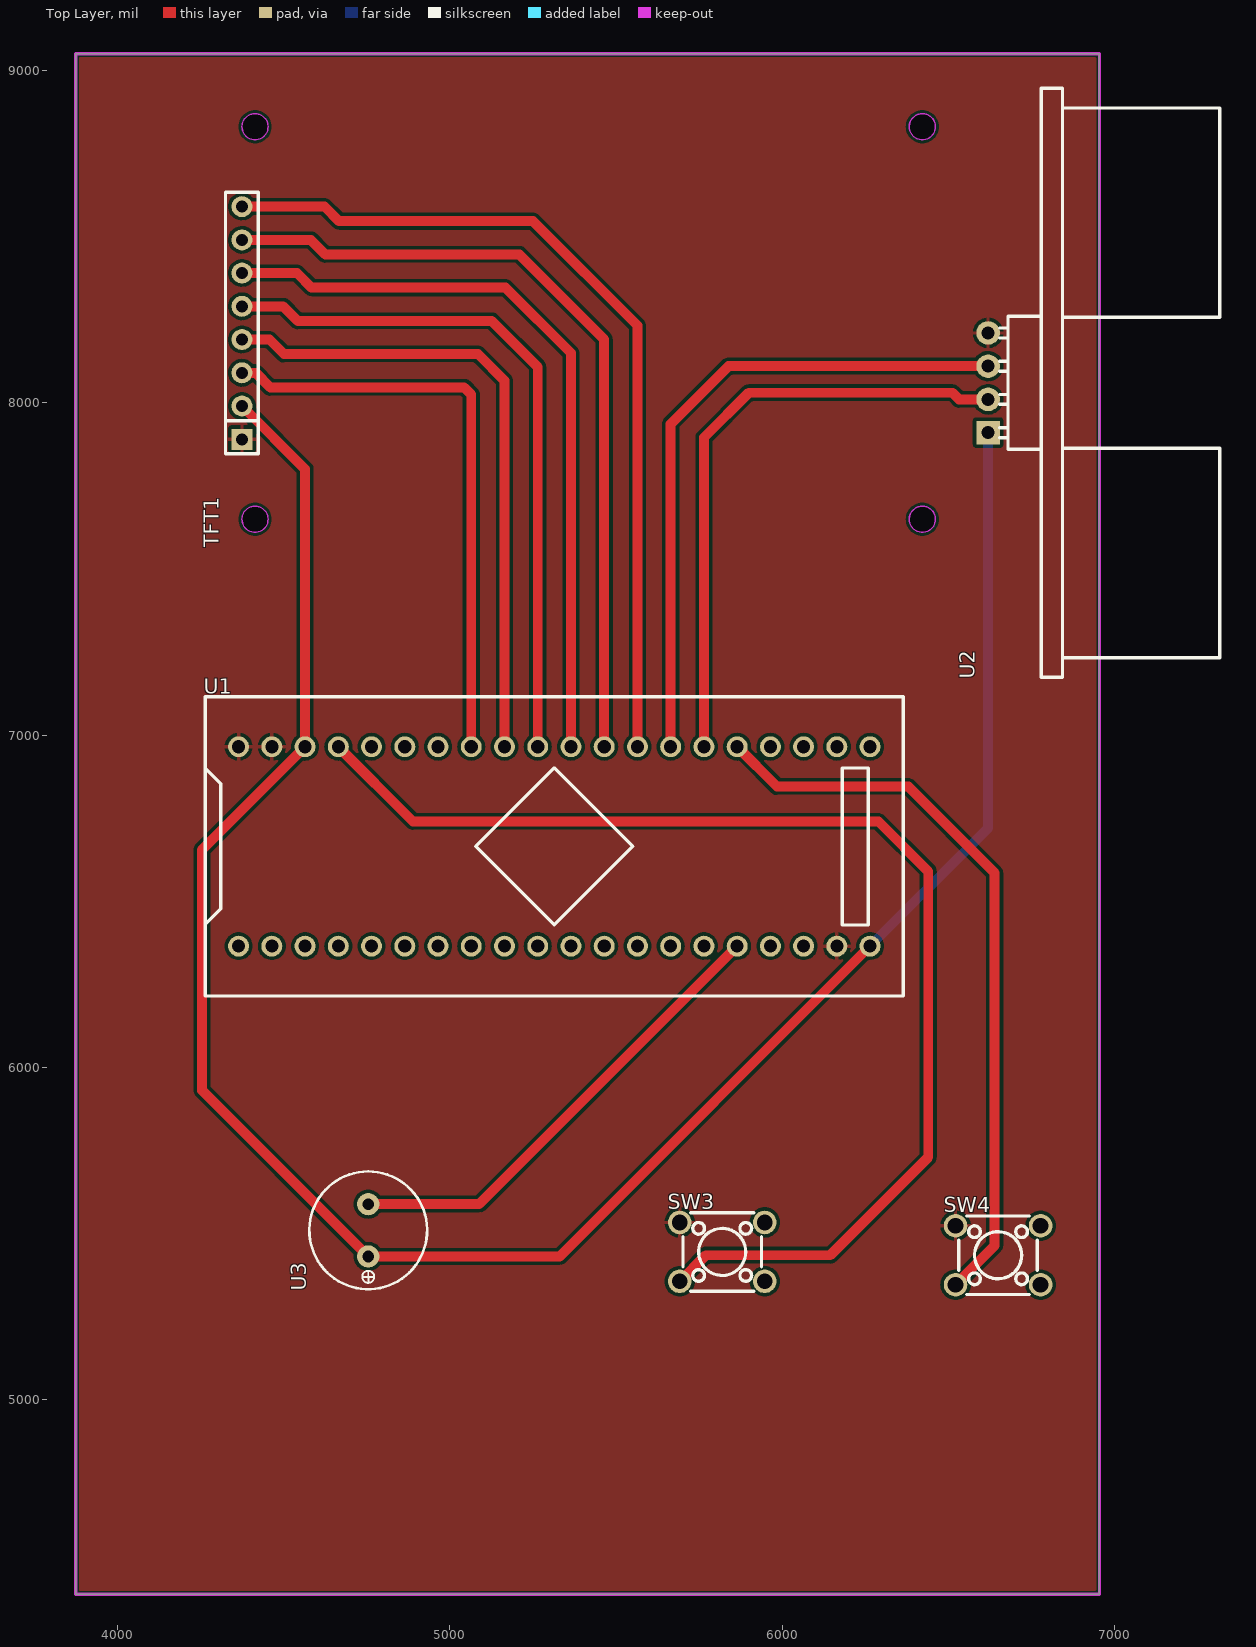
[diagram p0: Top Layer view]
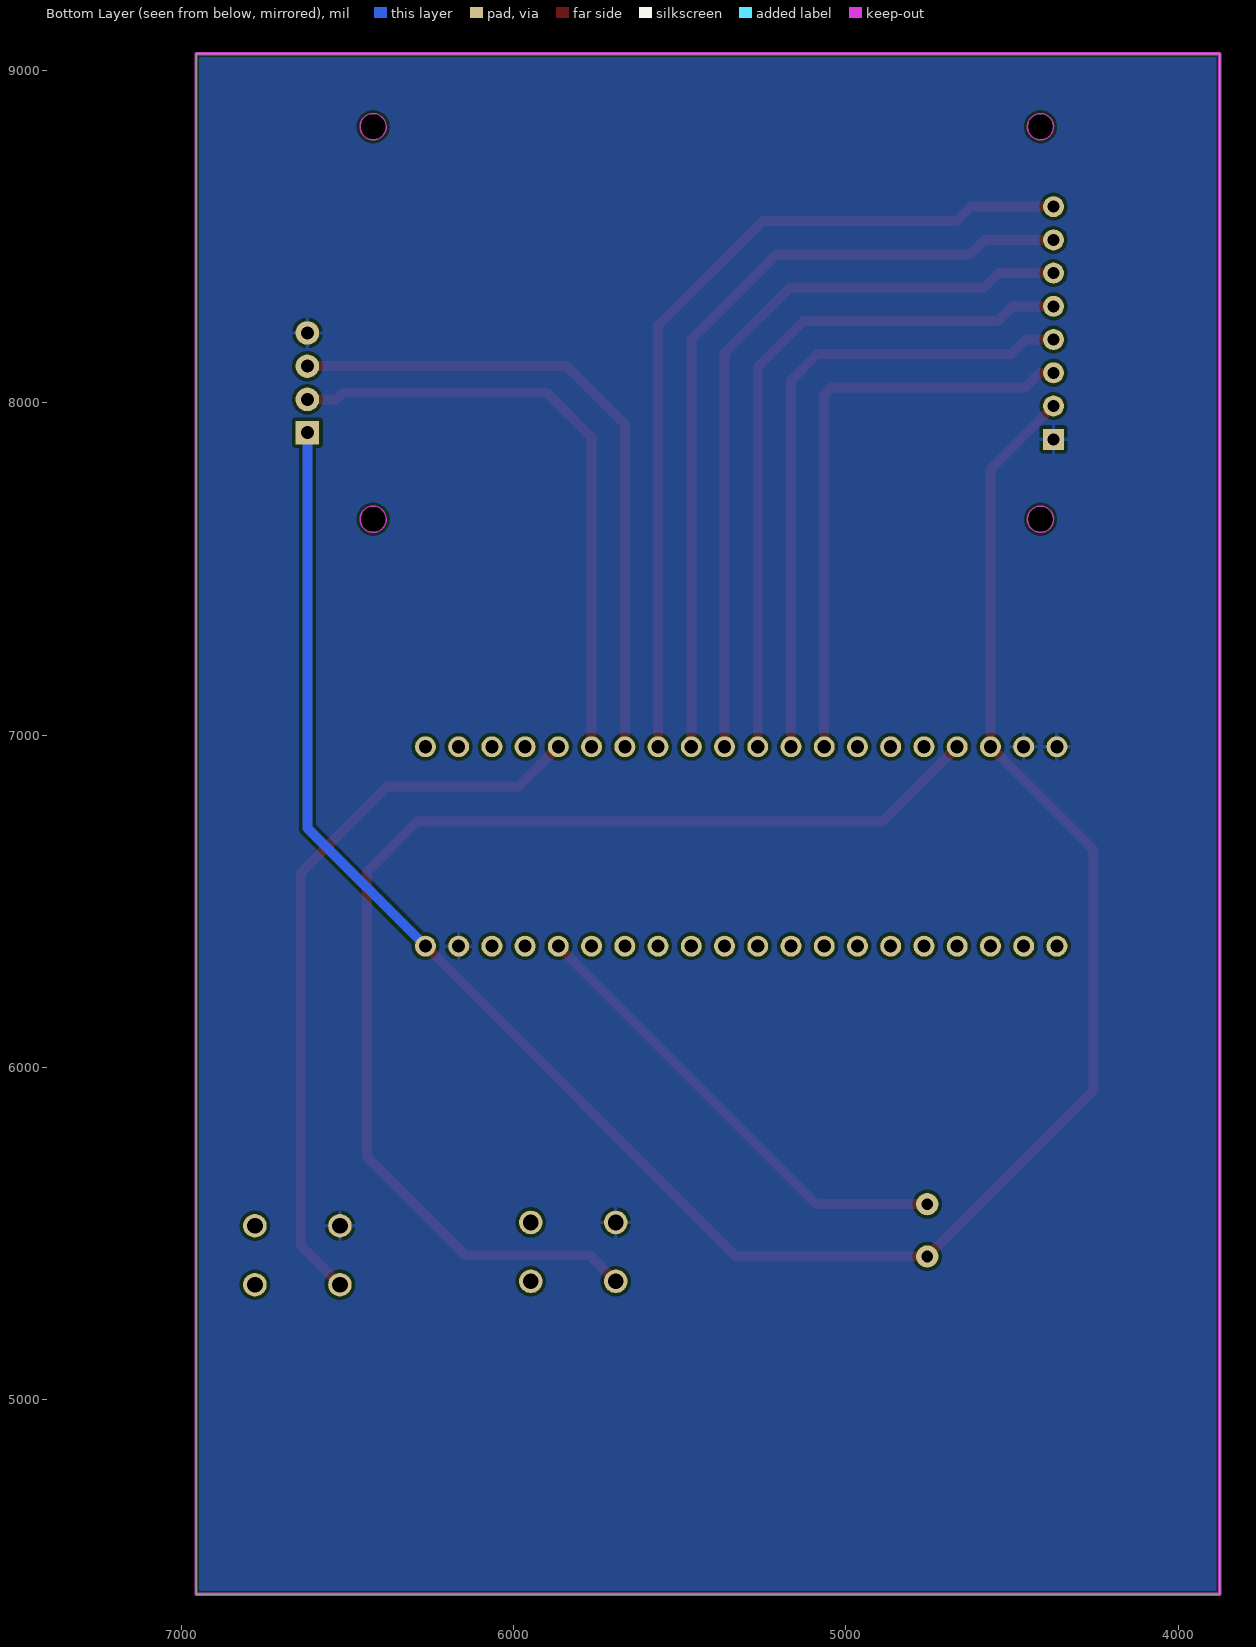
[diagram p1: Bottom Layer view, seen from below]
# Altium PCB MISC49920.pcbdoc
Units mil, origin at the board's own origin, x right, y up, seen from the top; angles counter-clockwise.
Board outline 3080 x 4635 mil, 2 copper layers (Top Layer, Bottom Layer), stack 62.206 mil thick; 6 components, 37 nets, 62 pads, 0 vias.

## Layer stack, top to bottom
Top Solder Mask Layer: solder mask 0.394, Dk 3.3
Top Layer: signal copper 1.379
Dielectric1: surface 59.449, FR4, Dk 4.5
Bottom Layer: signal copper 1.378
Bottom Solder Mask Layer: solder mask 0.394, Dk 3.3

## Board outline
3875,9050 3875,4415 6955,4415 6955,9050

## Design rules (kind name [scope] priority, off if disabled: settings)
BoardOutlineClearance copperThickness2oz_1 [All] p2 off: genericclearance=7.99 ignorepadtopadclearanceinfootprint=FALSE except(0: Arc-SplitContinuation Track-SplitContinuation SMDPad-SplitContinuation THPad-SplitContinuation Via-SplitContinuation Fill-SplitContinuation Region-SplitContinuation Poly-SplitContinuation Text-SplitContinuation Hole-SplitContinuation; 5.98: Arc-CutoutEdge Track-CutoutEdge SMDPad-CutoutEdge THPad-CutoutEdge Via-CutoutEdge Text-CutoutEdge; 6.9: Hole-OutlineEdge Hole-CutoutEdge; 10: Poly-OutlineEdge Poly-CutoutEdge; 11.81: Arc-OutlineEdge Track-OutlineEdge SMDPad-OutlineEdge THPad-OutlineEdge Via-OutlineEdge Fill-OutlineEdge Region-OutlineEdge Text-OutlineEdge Fill-CutoutEdge Region-CutoutEdge)
BoardOutlineClearance Plane_innerPlane_1 [All] p4 off: genericclearance=4.02 ignorepadtopadclearanceinfootprint=FALSE except(0: Arc-SplitContinuation Track-SplitContinuation SMDPad-SplitContinuation THPad-SplitContinuation Via-SplitContinuation Fill-SplitContinuation Region-SplitContinuation Poly-SplitContinuation Text-SplitContinuation Hole-SplitContinuation; 5.98: Arc-CutoutEdge Track-CutoutEdge SMDPad-CutoutEdge THPad-CutoutEdge Via-CutoutEdge Text-CutoutEdge; 6.9: Hole-OutlineEdge Hole-CutoutEdge; 10: Poly-OutlineEdge Poly-CutoutEdge; 11.81: Arc-OutlineEdge Track-OutlineEdge SMDPad-OutlineEdge THPad-OutlineEdge Via-OutlineEdge Fill-OutlineEdge Region-OutlineEdge Text-OutlineEdge Fill-CutoutEdge Region-CutoutEdge)
BoardOutlineClearance Copper_copperRegion_1 [All] p6 off: genericclearance=4.02 ignorepadtopadclearanceinfootprint=FALSE except(0: Arc-SplitContinuation Track-SplitContinuation SMDPad-SplitContinuation THPad-SplitContinuation Via-SplitContinuation Fill-SplitContinuation Region-SplitContinuation Poly-SplitContinuation Text-SplitContinuation Hole-SplitContinuation; 5.98: Arc-CutoutEdge Track-CutoutEdge SMDPad-CutoutEdge THPad-CutoutEdge Via-CutoutEdge Text-CutoutEdge; 6.9: Hole-OutlineEdge Hole-CutoutEdge; 10: Poly-OutlineEdge Poly-CutoutEdge; 11.81: Arc-OutlineEdge Track-OutlineEdge SMDPad-OutlineEdge THPad-OutlineEdge Via-OutlineEdge Fill-OutlineEdge Region-OutlineEdge Text-OutlineEdge Fill-CutoutEdge Region-CutoutEdge)
BoardOutlineClearance Copper_copperRegion_copperThickness1oz_1 [All] p8 off: genericclearance=4.02 ignorepadtopadclearanceinfootprint=FALSE except(0: Arc-SplitContinuation Track-SplitContinuation SMDPad-SplitContinuation THPad-SplitContinuation Via-SplitContinuation Fill-SplitContinuation Region-SplitContinuation Poly-SplitContinuation Text-SplitContinuation Hole-SplitContinuation; 5.98: Arc-CutoutEdge Track-CutoutEdge SMDPad-CutoutEdge THPad-CutoutEdge Via-CutoutEdge Text-CutoutEdge; 6.9: Hole-OutlineEdge Hole-CutoutEdge; 10: Poly-OutlineEdge Poly-CutoutEdge; 11.81: Arc-OutlineEdge Track-OutlineEdge SMDPad-OutlineEdge THPad-OutlineEdge Via-OutlineEdge Fill-OutlineEdge Region-OutlineEdge Text-OutlineEdge Fill-CutoutEdge Region-CutoutEdge)
BoardOutlineClearance Copper_copperRegion_Copper_copperRegion_1 [All] p10 off: genericclearance=4.02 ignorepadtopadclearanceinfootprint=FALSE except(0: Arc-SplitContinuation Track-SplitContinuation SMDPad-SplitContinuation THPad-SplitContinuation Via-SplitContinuation Fill-SplitContinuation Region-SplitContinuation Poly-SplitContinuation Text-SplitContinuation Hole-SplitContinuation; 5.98: Arc-CutoutEdge Track-CutoutEdge SMDPad-CutoutEdge THPad-CutoutEdge Via-CutoutEdge Text-CutoutEdge; 6.9: Hole-OutlineEdge Hole-CutoutEdge; 10: Poly-OutlineEdge Poly-CutoutEdge; 11.81: Arc-OutlineEdge Track-OutlineEdge SMDPad-OutlineEdge THPad-OutlineEdge Via-OutlineEdge Fill-OutlineEdge Region-OutlineEdge Text-OutlineEdge Fill-CutoutEdge Region-CutoutEdge)
BoardOutlineClearance copperThickness1oz_1 [All] p12: genericclearance=4.02 ignorepadtopadclearanceinfootprint=FALSE except(0: Arc-SplitContinuation Track-SplitContinuation SMDPad-SplitContinuation THPad-SplitContinuation Via-SplitContinuation Fill-SplitContinuation Region-SplitContinuation Poly-SplitContinuation Text-SplitContinuation Hole-SplitContinuation; 5.98: Arc-CutoutEdge Track-CutoutEdge SMDPad-CutoutEdge THPad-CutoutEdge Via-CutoutEdge Text-CutoutEdge; 6.9: Hole-OutlineEdge Hole-CutoutEdge; 10: Poly-OutlineEdge Poly-CutoutEdge; 11.81: Arc-OutlineEdge Track-OutlineEdge SMDPad-OutlineEdge THPad-OutlineEdge Via-OutlineEdge Fill-OutlineEdge Region-OutlineEdge Text-OutlineEdge Fill-CutoutEdge Region-CutoutEdge)
Clearance copperThickness2oz [All] p1 off: gap=7.99 ignorepadtopadclearanceinfootprint=FALSE except(5.98: SMDPad-Track SMDPad-SMDPad THPad-Track SMDPad-THPad THPad-THPad Track-Via SMDPad-Via THPad-Via Via-Via Fill-SMDPad Region-SMDPad Fill-THPad Region-THPad Fill-Via Region-Via Fill-Fill Fill-Region Region-Region Arc-Track Arc-SMDPad Arc-THPad Arc-Via Fill-Arc Region-Arc Arc-Arc Text-Track SMDPad-Text Text-THPad Text-Via Fill-Text Region-Text Arc-Text Text-Text; 6.9: Hole-Track Hole-SMDPad Hole-THPad Hole-Via Fill-Hole Region-Hole Hole-Arc Hole-Text; 10: Poly-Track Poly-SMDPad Poly-THPad Poly-Via Poly-Fill Poly-Region Poly-Poly Poly-Arc Poly-Text Poly-Hole; 11.81: Fill-Track Region-Track)
Clearance Plane_innerPlane [All] p3 off: gap=4.02 ignorepadtopadclearanceinfootprint=FALSE except(5.98: SMDPad-Track SMDPad-SMDPad THPad-Track SMDPad-THPad THPad-THPad Track-Via SMDPad-Via THPad-Via Via-Via Fill-SMDPad Region-SMDPad Fill-THPad Region-THPad Fill-Via Region-Via Fill-Fill Fill-Region Region-Region Arc-Track Arc-SMDPad Arc-THPad Arc-Via Fill-Arc Region-Arc Arc-Arc Text-Track SMDPad-Text Text-THPad Text-Via Fill-Text Region-Text Arc-Text Text-Text; 6.9: Hole-Track Hole-SMDPad Hole-THPad Hole-Via Fill-Hole Region-Hole Hole-Arc Hole-Text; 10: Poly-Track Poly-SMDPad Poly-THPad Poly-Via Poly-Fill Poly-Region Poly-Poly Poly-Arc Poly-Text Poly-Hole; 11.81: Fill-Track Region-Track)
Clearance Copper_copperRegion [All] p5 off: gap=4.02 ignorepadtopadclearanceinfootprint=FALSE except(5.98: SMDPad-Track SMDPad-SMDPad THPad-Track SMDPad-THPad THPad-THPad Track-Via SMDPad-Via THPad-Via Via-Via Fill-SMDPad Region-SMDPad Fill-THPad Region-THPad Fill-Via Region-Via Fill-Fill Fill-Region Region-Region Arc-Track Arc-SMDPad Arc-THPad Arc-Via Fill-Arc Region-Arc Arc-Arc Text-Track SMDPad-Text Text-THPad Text-Via Fill-Text Region-Text Arc-Text Text-Text; 6.9: Hole-Track Hole-SMDPad Hole-THPad Hole-Via Fill-Hole Region-Hole Hole-Arc Hole-Text; 10: Poly-Track Poly-SMDPad Poly-THPad Poly-Via Poly-Fill Poly-Region Poly-Poly Poly-Arc Poly-Text Poly-Hole; 11.81: Fill-Track Region-Track)
Clearance Copper_copperRegion_copperThickness1oz [All] p7 off: gap=4.02 ignorepadtopadclearanceinfootprint=FALSE except(5.98: SMDPad-Track SMDPad-SMDPad THPad-Track SMDPad-THPad THPad-THPad Track-Via SMDPad-Via THPad-Via Via-Via Fill-SMDPad Region-SMDPad Fill-THPad Region-THPad Fill-Via Region-Via Fill-Fill Fill-Region Region-Region Arc-Track Arc-SMDPad Arc-THPad Arc-Via Fill-Arc Region-Arc Arc-Arc Text-Track SMDPad-Text Text-THPad Text-Via Fill-Text Region-Text Arc-Text Text-Text; 6.9: Hole-Track Hole-SMDPad Hole-THPad Hole-Via Fill-Hole Region-Hole Hole-Arc Hole-Text; 10: Poly-Track Poly-SMDPad Poly-THPad Poly-Via Poly-Fill Poly-Region Poly-Poly Poly-Arc Poly-Text Poly-Hole; 11.81: Fill-Track Region-Track)
Clearance Copper_copperRegion_Copper_copperRegion [All] p9 off: gap=4.02 ignorepadtopadclearanceinfootprint=FALSE except(5.98: SMDPad-Track SMDPad-SMDPad THPad-Track SMDPad-THPad THPad-THPad Track-Via SMDPad-Via THPad-Via Via-Via Fill-SMDPad Region-SMDPad Fill-THPad Region-THPad Fill-Via Region-Via Fill-Fill Fill-Region Region-Region Arc-Track Arc-SMDPad Arc-THPad Arc-Via Fill-Arc Region-Arc Arc-Arc Text-Track SMDPad-Text Text-THPad Text-Via Fill-Text Region-Text Arc-Text Text-Text; 6.9: Hole-Track Hole-SMDPad Hole-THPad Hole-Via Fill-Hole Region-Hole Hole-Arc Hole-Text; 10: Poly-Track Poly-SMDPad Poly-THPad Poly-Via Poly-Fill Poly-Region Poly-Poly Poly-Arc Poly-Text Poly-Hole; 11.81: Fill-Track Region-Track)
Clearance copperThickness1oz [All] p11: gap=4.02 ignorepadtopadclearanceinfootprint=FALSE except(5.98: SMDPad-Track SMDPad-SMDPad THPad-Track SMDPad-THPad THPad-THPad Track-Via SMDPad-Via THPad-Via Via-Via Fill-SMDPad Region-SMDPad Fill-THPad Region-THPad Fill-Via Region-Via Fill-Fill Fill-Region Region-Region Arc-Track Arc-SMDPad Arc-THPad Arc-Via Fill-Arc Region-Arc Arc-Arc Text-Track SMDPad-Text Text-THPad Text-Via Fill-Text Region-Text Arc-Text Text-Text; 6.9: Hole-Track Hole-SMDPad Hole-THPad Hole-Via Fill-Hole Region-Hole Hole-Arc Hole-Text; 10: Poly-Track Poly-SMDPad Poly-THPad Poly-Via Poly-Fill Poly-Region Poly-Poly Poly-Arc Poly-Text Poly-Hole; 11.81: Fill-Track Region-Track)
DiffPairsRouting differentialPair [All] p1: maxlimit=6 minlimit=6 mostfreqgap=6 toplayer_minwidth=5 toplayer_prefwidth=10 toplayer_maxwidth=100 toplayer_mingap=6 toplayer_prefgap=6 toplayer_maxgap=6 bottomlayer_minwidth=5 bottomlayer_prefwidth=10 bottomlayer_maxwidth=100 bottomlayer_mingap=6 bottomlayer_prefgap=6 bottomlayer_maxgap=6 maxuncoupledlength=10
HoleToHoleClearance otherClearance [All] p1: gap=11.81 allowstackedmicrovias=TRUE
Length netLength [All] p1: minlimit=0 maxlimit=0
PasteMaskExpansion pasteMaskExpansion [All] p1: expansion=0
PlaneConnect innerPlane [All] p1: planeconnectstyle=Relief reliefexpansion=20 reliefentries=4 reliefconductorwidth=10 reliefairgap=10
PolygonConnect copperRegion_copperThickness1oz [(InNet('GND'))] p1: connectstyle=Relief reliefconductorwidth=10 reliefentries=4 polygonreliefangle="90 Angle" airgapwidth=10 via.connectstyle=Relief via.reliefconductorwidth=10 via.reliefentries=4 via.polygonreliefangle="90 Angle" via.airgapwidth=10
PolygonConnect copperRegion_Copper_copperRegion [All] p2 off: connectstyle=Relief reliefconductorwidth=10 reliefentries=4 polygonreliefangle="90 Angle" airgapwidth=10 via.connectstyle=Relief via.reliefconductorwidth=10 via.reliefentries=4 via.polygonreliefangle="90 Angle" via.airgapwidth=10
PolygonConnect copperRegion [All] p3: connectstyle=Relief reliefconductorwidth=10 reliefentries=4 polygonreliefangle="90 Angle" airgapwidth=10 via.connectstyle=Relief via.reliefconductorwidth=10 via.reliefentries=4 via.polygonreliefangle="90 Angle" via.airgapwidth=10
RoutingVias viaSize [All] p1: holewidth=12.01 width=24.02 viastyle="Through Hole" minholewidth=11.81 minwidth=19.68 maxholewidth=248.03 maxwidth=393.7
SolderMaskExpansion solderMaskExpansion [IsVia] p1: expansion=-1000 istentingtop=TRUE
SolderMaskExpansion solderMaskExpansion [All] p2: expansion=2 istentingtop=FALSE
Width copperThickness2oz_2 [All] p1 off: maxlimit=100 minlimit=8 preferedwidth=10
Width copperThickness1oz_2 [All] p2: maxlimit=100 minlimit=5 preferedwidth=10

## Components (designator, comment, footprint, x,y, rotation, side; value= is the part's Value field where it differs from the comment)
SW3 "" SW-TH_4P-L6.0-W6.0-P4.50-LS6.5 5820,5445 r0 top
SW4 "" SW-TH_4P-L6.0-W6.0-P4.50-LS6.5 6650,5435 r0 top
TFT1 "1.8 TFT 128*RGB*160" LCD-TH_8P-P2.54-L56.0-W34.0_1.8-TFT 4375,8240 r90 top
U1 "STM32F103C8T6-Card" CONN-TH_L53.3-W22.9_STM32F103C8T6-CARD 5315,6665 r0 top
U2 "HC-SR04" TH_HC-SR04V 6620,8060 r90 top
U3 "CUI_CST-931AP" BUZ-TH_BD9.0-P4.00-D0.6-L-FD 4755,5510 r90 top

## Footprints (in the part's own frame and the unit in brackets; to place one, negate y for a bottom-side part, rotate by r counter-clockwise, add the part's x,y. Pads: shape width x height; smd on the part's side, far side on the other; paste and mask are expansions set on the pad)
BUZ-TH_BD9.0-P4.00-D0.6-L-FD [mm]
  round 1.7 hole 0.9 paste+0 mask+0.05: 1(-2,0) 2(2,0)
  silkscreen extent -4.5,-4.5 4.5,4.5
CONN-TH_L53.3-W22.9_STM32F103C8T6-CARD [mm]
  round 1.6 hole 1: 1(-24.13,-7.62) 2(-21.59,-7.62) 3(-19.05,-7.62) 4(-16.51,-7.62) 5(-13.97,-7.62) 6(-11.43,-7.62) 7(-8.89,-7.62) 8(-6.35,-7.62) 9(-3.81,-7.62) 10(-1.27,-7.62) 11(1.27,-7.62) 12(3.81,-7.62) 13(6.35,-7.62) 14(8.89,-7.62) 15(11.43,-7.62) 16(13.97,-7.62) 17(16.51,-7.62) 18(19.05,-7.62) 19(21.59,-7.62) 20(24.13,-7.62) 21(24.13,7.62) 22(21.59,7.62) 23(19.05,7.62) 24(16.51,7.62) 25(13.97,7.62) 26(11.43,7.62) 27(8.89,7.62) 28(6.35,7.62) 29(3.81,7.62) 30(1.27,7.62) 31(-1.27,7.62) 32(-3.81,7.62) 33(-6.35,7.62) 34(-8.89,7.62) 35(-11.43,7.62) 36(-13.97,7.62) 37(-16.51,7.62) 38(-19.05,7.62) 39(-21.59,7.62) 40(-24.13,7.62)
  silkscreen extent -26.67,-11.43 26.67,11.43
LCD-TH_8P-P2.54-L56.0-W34.0_1.8-TFT [mm]
  rect 1.6x1.6 hole 0.914: 1(-8.89,0)
  round 1.6 hole 0.914: 2(-6.35,0) 3(-3.81,0) 4(-1.27,0) 5(1.27,0) 6(3.81,0) 7(6.35,0) 8(8.89,0)
  Board Outline Layer circle w0.003: c15,-1 r1
  Board Outline Layer circle w0.003: c-15,-1 r1
  Board Outline Layer circle w0.003: c15,-52 r1
  Board Outline Layer circle w0.003: c-15,-52 r1
  Board Outline Layer region: 15,-2 14.566,-1.901 14.218,-1.623 14.025,-1.223 14.025,-0.777 14.218,-0.377 14.566,-0.099 15,0 15,0 15.434,-0.099 15.782,-0.377 15.975,-0.777 15.975,-1.223 15.782,-1.623 15.434,-1.901 15,-2
  Board Outline Layer region: 15,-2 14.864,-1.991 14.73,-1.963 14.602,-1.917 14.48,-1.854 14.369,-1.776 14.269,-1.683 14.183,-1.577 14.112,-1.46 14.058,-1.335 14.021,-1.203 14.002,-1.068 14.002,-0.932 14.021,-0.797 14.058,-0.665 14.112,-0.54 14.183,-0.423 14.269,-0.317 14.369,-0.224 14.48,-0.146 14.602,-0.083 14.73,-0.037 14.864,-0.009 15,0 15.136,-0.009 15.27,-0.037 15.398,-0.083 15.52,-0.146 15.631,-0.224 15.731,-0.317 15.817,-0.423 15.888,-0.54 15.942,-0.665 15.979,-0.797 15.998,-0.932 15.998,-1.068 15.979,-1.203 15.942,-1.335 15.888,-1.46 15.817,-1.577 15.731,-1.683 15.631,-1.776 15.52,-1.854 15.398,-1.917 15.27,-1.963 15.136,-1.991
  Board Outline Layer region: -15,-2 -15.434,-1.901 -15.782,-1.623 -15.975,-1.223 -15.975,-0.777 -15.782,-0.377 -15.434,-0.099 -15,0 -15,0 -14.566,-0.099 -14.218,-0.377 -14.025,-0.777 -14.025,-1.223 -14.218,-1.623 -14.566,-1.901 -15,-2
  Board Outline Layer region: -15,-2 -15.136,-1.991 -15.27,-1.963 -15.398,-1.917 -15.52,-1.854 -15.631,-1.776 -15.731,-1.683 -15.817,-1.577 -15.888,-1.46 -15.942,-1.335 -15.979,-1.203 -15.998,-1.068 -15.998,-0.932 -15.979,-0.797 -15.942,-0.665 -15.888,-0.54 -15.817,-0.423 -15.731,-0.317 -15.631,-0.224 -15.52,-0.146 -15.398,-0.083 -15.27,-0.037 -15.136,-0.009 -15,0 -14.864,-0.009 -14.73,-0.037 -14.602,-0.083 -14.48,-0.146 -14.369,-0.224 -14.269,-0.317 -14.183,-0.423 -14.112,-0.54 -14.058,-0.665 -14.021,-0.797 -14.002,-0.932 -14.002,-1.068 -14.021,-1.203 -14.058,-1.335 -14.112,-1.46 -14.183,-1.577 -14.269,-1.683 -14.369,-1.776 -14.48,-1.854 -14.602,-1.917 -14.73,-1.963 -14.864,-1.991
  Board Outline Layer region: 15,-53 14.566,-52.901 14.218,-52.623 14.025,-52.222 14.025,-51.777 14.218,-51.376 14.566,-51.099 15,-51 15,-51 15.434,-51.099 15.782,-51.376 15.975,-51.777 15.975,-52.222 15.782,-52.623 15.434,-52.901 15,-53
  Board Outline Layer region: 15,-53 14.864,-52.991 14.73,-52.963 14.602,-52.917 14.48,-52.854 14.369,-52.776 14.269,-52.682 14.183,-52.577 14.112,-52.46 14.058,-52.335 14.021,-52.203 14.002,-52.068 14.002,-51.932 14.021,-51.796 14.058,-51.665 14.112,-51.54 14.183,-51.423 14.269,-51.317 14.369,-51.224 14.48,-51.145 14.602,-51.083 14.73,-51.037 14.864,-51.009 15,-51 15.136,-51.009 15.27,-51.037 15.398,-51.083 15.52,-51.145 15.631,-51.224 15.731,-51.317 15.817,-51.423 15.888,-51.54 15.942,-51.665 15.979,-51.796 15.998,-51.932 15.998,-52.068 15.979,-52.203 15.942,-52.335 15.888,-52.46 15.817,-52.577 15.731,-52.682 15.631,-52.776 15.52,-52.854 15.398,-52.917 15.27,-52.963 15.136,-52.991
  Board Outline Layer region: -15,-53 -15.434,-52.901 -15.782,-52.623 -15.975,-52.222 -15.975,-51.777 -15.782,-51.376 -15.434,-51.099 -15,-51 -15,-51 -14.566,-51.099 -14.218,-51.376 -14.025,-51.777 -14.025,-52.222 -14.218,-52.623 -14.566,-52.901 -15,-53
  Board Outline Layer region: -15,-53 -15.136,-52.991 -15.27,-52.963 -15.398,-52.917 -15.52,-52.854 -15.631,-52.776 -15.731,-52.682 -15.817,-52.577 -15.888,-52.46 -15.942,-52.335 -15.979,-52.203 -15.998,-52.068 -15.998,-51.932 -15.979,-51.796 -15.942,-51.665 -15.888,-51.54 -15.817,-51.423 -15.731,-51.317 -15.631,-51.224 -15.52,-51.145 -15.398,-51.083 -15.27,-51.037 -15.136,-51.009 -15,-51 -14.864,-51.009 -14.73,-51.037 -14.602,-51.083 -14.48,-51.145 -14.369,-51.224 -14.269,-51.317 -14.183,-51.423 -14.112,-51.54 -14.058,-51.665 -14.021,-51.796 -14.002,-51.932 -14.002,-52.068 -14.021,-52.203 -14.058,-52.335 -14.112,-52.46 -14.183,-52.577 -14.269,-52.682 -14.369,-52.776 -14.48,-52.854 -14.602,-52.917 -14.73,-52.963 -14.864,-52.991
  Multi-Layer board cut-out: 15,-2 14.566,-1.901 14.218,-1.623 14.025,-1.223 14.025,-0.777 14.218,-0.377 14.566,-0.099 15,0 15,0 15.434,-0.099 15.782,-0.377 15.975,-0.777 15.975,-1.223 15.782,-1.623 15.434,-1.901 15,-2
  Multi-Layer board cut-out: -15,-2 -15.434,-1.901 -15.782,-1.623 -15.975,-1.223 -15.975,-0.777 -15.782,-0.377 -15.434,-0.099 -15,0 -15,0 -14.566,-0.099 -14.218,-0.377 -14.025,-0.777 -14.025,-1.223 -14.218,-1.623 -14.566,-1.901 -15,-2
  Multi-Layer board cut-out: 15,-53 14.566,-52.901 14.218,-52.623 14.025,-52.222 14.025,-51.777 14.218,-51.376 14.566,-51.099 15,-51 15,-51 15.434,-51.099 15.782,-51.376 15.975,-51.777 15.975,-52.222 15.782,-52.623 15.434,-52.901 15,-53
  Multi-Layer board cut-out: -15,-53 -15.434,-52.901 -15.782,-52.623 -15.975,-52.222 -15.975,-51.777 -15.782,-51.376 -15.434,-51.099 -15,-51 -15,-51 -14.566,-51.099 -14.218,-51.376 -14.025,-51.777 -14.025,-52.222 -14.218,-52.623 -14.566,-52.901 -15,-53
  silkscreen extent -10,-1.25 10,1.25
SW-TH_4P-L6.0-W6.0-P4.50-LS6.5 [mm]
  round 1.8 hole 1.2: 1(-3.25,2.25) 2(3.25,2.25) 3(-3.25,-2.25) 4(3.25,-2.25)
  silkscreen extent -3,-3 3,3
TH_HC-SR04V [mm]
  rect 1.8x1.8 hole 1.001: 1(-3.81,0)
  round 1.8 hole 1.001: 2(-1.27,0) 3(1.27,0) 4(3.81,0)
  silkscreen extent -22.5,-17.7 22.5,-0.89

## Nets (pads, with @x,y where several pads share a name; then routed paths per layer and width w, separated by ;. In a path a pad name is that pad's centre, name@x,y a point inside that pad or via, vN(x,y) a via of type N, cw(c..) or ccw(c..) an arc to the next point about the centre after c; other vN are vias at no path point)
+5V: U1.18
GND: SW3.1 SW4.1 TFT1.1 U1.19 U1.39 U1.40 U2.4
NRST: SW3.3 U1.37 | length 3693
  Top Layer w30: U1.37 4890,6740 6290,6740 6440,6590 6440,5730 6145,5435 5770.63,5435 SW3.3
PA0: SW4.3 U1.25 | length 2219.8
  Top Layer w30: U1.25 5985,6845 6380,6845 6640,6585 6640,5464.37 SW4.3
PA1: U1.26 U2.2 | length 1849.2
  Top Layer w30: U1.26 5765,7895 5900,8030 6513.15,8030 6533.15,8010 U2.2
PA2: U1.27 U2.3 | length 1998.3
  Top Layer w30: U1.27 5665,7936.42 5838.58,8110 U2.3
PA3: TFT1.8 U1.28 | length 2605.4
  Top Layer w30: TFT1.8 4623.6,8590 4667.39,8546.21 5250.9,8546.21 5565,8232.11 U1.28
PA4: TFT1.7 U1.29 | length 2439.7
  Top Layer w30: TFT1.7 4582.18,8490 4625.97,8446.21 5209.47,8446.21 5465,8190.69 U1.29
PA5: TFT1.6 U1.30 | length 2274
  Top Layer w30: TFT1.6 4540.76,8390 4584.55,8346.21 5168.05,8346.21 5365,8149.26 U1.30
PA6: TFT1.5 U1.31 | length 2108.3
  Top Layer w30: TFT1.5 4499.34,8290 4543.13,8246.21 5126.63,8246.21 5265,8107.84 U1.31
PA7: TFT1.4 U1.32 | length 1942.6
  Top Layer w30: TFT1.4 4457.92,8190 4501.7,8146.21 5085.21,8146.21 5165,8066.42 U1.32
PA8: U1.5
PA9: U1.6
PA10: U1.7
PA11: U1.8
PA12: U1.9
PA15: U1.10
PB0: TFT1.3 U1.33 | length 1776.9
  Top Layer w30: TFT1.3 4416.5,8090 4460.28,8046.21 5043.79,8046.21 5065,8025 U1.33
PB1: U1.34
PB3: U1.11
PB4: U1.12
PB5: U1.13
PB6: U1.14
PB7: U1.15
PB8: U1.16 U3.2 | length 1431.5
  Top Layer w30: U3.2 5088.74,5588.74 U1.16
PB9: U1.17
PB10: U1.35
PB11: U1.36
PB12: U1.1
PB13: U1.2
PB14: U1.3
PB15: U1.4
PC13: U1.22
PC14: U1.23
PC15: U1.24
VBAT: U1.21
VCC: TFT1.2 U1.20 U1.38 U2.1 U3.1 | length 6561.8
  Top Layer w30: TFT1.2 4565,7800 U1.38 4255,6655 4255,5931.26 U3.1 5331.26,5431.26 U1.20
  Bottom Layer w30: U1.20 6620,6720 U2.1
pads on no net: SW3.2 SW3.4 SW4.2 SW4.4

## Polygon pours and split planes (outlines as drawn)
GND on Bottom Layer (solid, remove dead copper, pour order 2): 3345,9725 3345,3000 8540,3000 8540,9725
GND on Top Layer (solid, remove dead copper, pour order 0): 3000,9670 3000,3930 7995,3930 7995,9670

## Keep-outs
Board Outline Layer:
  the board outline again, w10